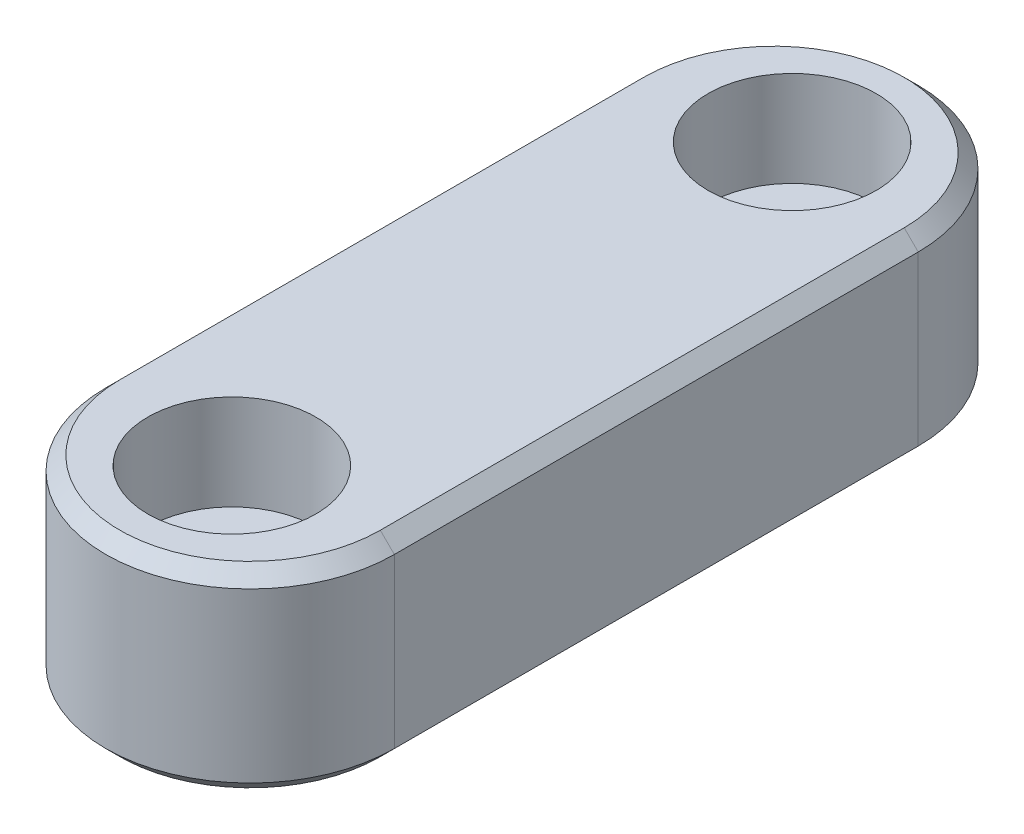
from build123d import *

# Parameters (mm, degrees)
SKETCH1_W                                           = 10.3
SKETCH1_H                                           = 7
BOSS_EXTRUDE1_DEPTH                                 = 29
FILLET1_RADIUS                                      = 5.15
FILLET1_LENGTH                                      = 7
FILLET2_RADIUS                                      = 5.15
FILLET2_LENGTH                                      = 7
CHAMFER1_SIZE                                       = 0.5
HOLE_SPEC_PER_SOCKET_HEAD_CAP_SCREW_TYP_D           = 3.4
HOLE_SPEC_PER_SOCKET_HEAD_CAP_SCREW_TYP_CBORE_D     = 6
HOLE_SPEC_PER_SOCKET_HEAD_CAP_SCREW_TYP_CBORE_DEPTH = 3.4


with BuildPart() as part:
    # Sketch1 → Boss-Extrude1 (new body)
    with BuildSketch(Plane.XY):
        Rectangle(SKETCH1_W, SKETCH1_H)
    extrude(amount=BOSS_EXTRUDE1_DEPTH)

    # Fillet1: full round fillet: the end face becomes a half cylinder, R = half its width
    fillet1_face = Plane((0, 0, 0), x_dir=(0, 1, 0), z_dir=(0, 0, -1))  # on the end face: x along it, z out of the body
    fillet1_slab = fillet1_face.offset(-FILLET1_RADIUS / 2) * Box(FILLET1_LENGTH, 2 * FILLET1_RADIUS, FILLET1_RADIUS, mode=Mode.PRIVATE)  # the body's end, R deep
    fillet1_round = Plane((0, 0, 5.15), x_dir=(0, 0, -1), z_dir=(0, 1, 0)) * Cylinder(FILLET1_RADIUS, FILLET1_LENGTH, mode=Mode.PRIVATE)  # its axis R under the face
    add(fillet1_slab - fillet1_round, mode=Mode.SUBTRACT)

    # Fillet2: full round fillet: the end face becomes a half cylinder, R = half its width
    fillet2_face = Plane((0, 0, 29), x_dir=(0, -1, 0), z_dir=(0, 0, 1))  # on the end face: x along it, z out of the body
    fillet2_slab = fillet2_face.offset(-FILLET2_RADIUS / 2) * Box(FILLET2_LENGTH, 2 * FILLET2_RADIUS, FILLET2_RADIUS, mode=Mode.PRIVATE)  # the body's end, R deep
    fillet2_round = Plane((0, 0, 23.85), x_dir=(0, 0, 1), z_dir=(0, -1, 0)) * Cylinder(FILLET2_RADIUS, FILLET2_LENGTH, mode=Mode.PRIVATE)  # its axis R under the face
    add(fillet2_slab - fillet2_round, mode=Mode.SUBTRACT)

    # Chamfer1
    chamfer1_edges = [part.edges().sort_by_distance(p)[0] for p in [
        (0, -3.5, 0),
        (0, 3.5, 0),
        (5.15, -3.5, 14.5),
        (5.15, 3.5, 14.5),
        (-5.15, 3.5, 14.5),
        (-5.15, -3.5, 14.5),
        (0, 3.5, 29),
        (0, -3.5, 29),
    ]]
    chamfer(chamfer1_edges, length=CHAMFER1_SIZE)

    # Hole Spec (per socket head cap screw type) 1 (through all)
    with Locations(Plane(origin=(0, 3.5, 0), x_dir=(1, 0, 0), z_dir=(0, 1, 0))):
        with Locations((0, -24.5), (0, -4.5)):
            CounterBoreHole(HOLE_SPEC_PER_SOCKET_HEAD_CAP_SCREW_TYP_D / 2, HOLE_SPEC_PER_SOCKET_HEAD_CAP_SCREW_TYP_CBORE_D / 2, HOLE_SPEC_PER_SOCKET_HEAD_CAP_SCREW_TYP_CBORE_DEPTH)


solid = part.part
